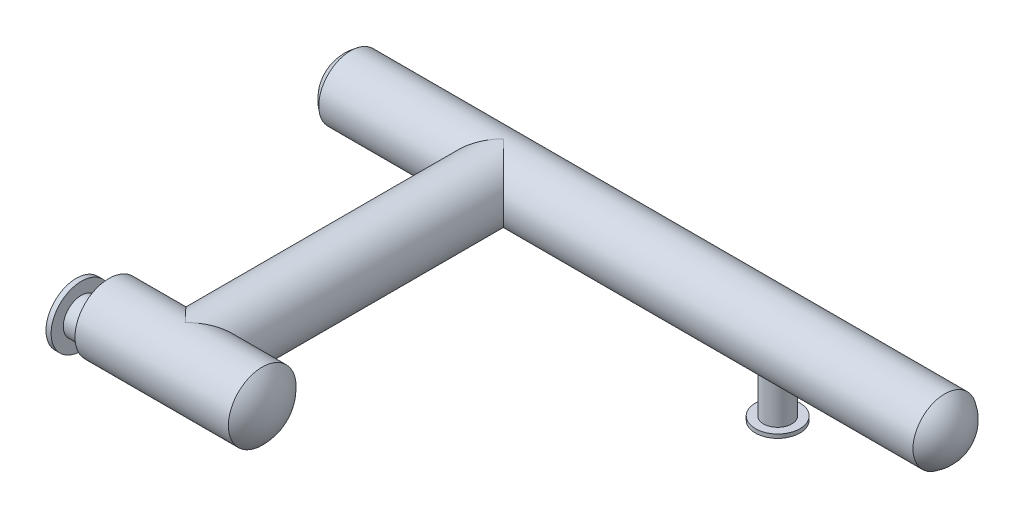
SolidWorks part; units mm, degrees
material "普通碳钢"
ref_plane "Front Plane" through (0, 0, 0) normal (0, 0, 1) x (1, 0, 0)
ref_plane "Top Plane" through (0, 0, 0) normal (0, 1, 0) x (1, 0, 0)
ref_plane "Right Plane" through (0, 0, 0) normal (1, 0, 0) x (0, 0, -1)
sketch "Sketch1" plane through (0, 0, 0) normal (0, 0, 1) x (1, 0, 0)
  line L5 (159.8445, 150) -> (2962.0029, 150)
  line L16 (0, 0) -> (89.3432, 0) construction
  line L17 (79.3432, 0) -> (89.3432, 0)
  line L18 (3047.486, 0) -> (3037.486, 0)
  line L19 (3047.486, 0) -> (2990.0914, 0) construction
  line L20 (162.9067, 140) -> (2959.2196, 140)
  line L21 (96.2314, 0) -> (389.3753, 0) construction
  line L22 (3037.1815, 10) -> (2990.0914, 10) construction
  line L23 (89.6376, 10) -> (96.2314, 10) construction
  line L24 (79.3432, 0) -> (96.2314, 0) construction
  arc A0 (159.8445, 150) -> (79.3432, 0) centre (259.3432, 0) ccw
  arc A1 (2962.0029, 150) -> (3047.486, 0) centre (2873.1395, 0) cw
  arc A2 (2959.2196, 140) -> (3037.486, 0) centre (2873.1395, 0) cw
  arc A3 (162.9067, 140) -> (89.3432, 0) centre (259.3432, 0) ccw
  arc A4 (2959.2196, 140) -> (3037.1815, 10) centre (2873.1395, 0) cw construction
  arc A5 (162.9067, 140) -> (89.6376, 10) centre (259.3432, 0) ccw construction
  dimension "D2" = 180
  dimension "D1" = 10
  dimension "D3" = 150
revolve "Revolve1" add sketch "Sketch1" angle 360 about L16
sketch "Sketch2" plane through (0, 0, 0) normal (0, 0, 1) x (1, 0, 0)
  circle A0 centre (880, 0) radius 150
  circle A1 centre (880, 0) radius 140
  dimension "D1" = 300
  dimension "D2" = 10
extrude "Boss-Extrude1" add sketch "Sketch2" along normal blind 1500
ref_plane "Plane1" through (0, 0, 1500) normal (0, 0, 1) x (1, 0, 0)
sketch "Sketch4" plane through (0, 0, 1500) normal (0, 0, 1) x (1, 0, 0)
  line L1 (1243.1971, 150) -> (519.9222, 150)
  line L2 (2962.0029, 150) -> (880, 150) construction
  line L3 (880, 150) -> (159.8445, 150) construction
  line L4 (496.4048, -9.7617) -> (506.4058, -9.7617)
  line L8 (1239.1001, 140) -> (527.5168, 140)
  line L10 (506.6346, 0.2383) -> (1299.0754, 0.2383) construction
  line L11 (1299.1071, -9.7617) -> (1309.1092, -9.7617)
  line L12 (496.4048, -9.7617) -> (1309.1092, -9.7617) construction
  arc A1 (1309.1092, -9.7617) -> (1243.1971, 150) centre (1093.0729, -5.4133) ccw
  arc A2 (496.4048, -9.7617) -> (519.9222, 150) centre (1110.7572, -18.5847) cw
  arc A3 (506.4058, -9.7617) -> (527.5168, 140) centre (1110.7572, -18.5847) cw
  arc A4 (1299.1071, -9.7617) -> (1239.1001, 140) centre (1093.0729, -5.4133) ccw
  arc A5 (506.6346, 0.2383) -> (527.5168, 140) centre (1110.7572, -18.5847) cw construction
  arc A6 (1299.0754, 0.2383) -> (1239.1001, 140) centre (1093.0729, -5.4133) ccw construction
  dimension "D2" = 10
revolve "Revolve2" add sketch "Sketch4" angle 360 about L4
ref_plane "Plane2" through (550, 0, 0) normal (1, 0, 0) x (0, 0, -1)
sketch "Sketch5" plane through (550, 0, 0) normal (1, 0, 0) x (0, 0, -1)
  circle A0 centre (-1559.9921, -8.7899) radius 85
  circle A1 centre (-1559.9921, -8.7899) radius 79
  circle A2 centre (-1500, -9.7617) radius 159.7617 construction
  dimension "D1" = 170
  dimension "D2" = 6
  dimension "D3" = 60
extrude "Boss-Extrude2" add sketch "Sketch5" against normal blind 100 separate body
sketch "Sketch6" plane through (450, 0, 0) normal (-1, 0, 0) x (0, 0, 1)
  circle A0 centre (1559.9921, -8.7899) radius 60.5
  circle A1 centre (1559.9921, -8.7899) radius 142.5
  dimension "D1" = 285
extrude "Boss-Extrude3" add sketch "Sketch6" along normal blind 24
sketch "Sketch9" plane through (0, 0, 0) normal (0, 1, 0) x (1, 0, 0)
  line L0 (2962.0029, -150) -> (2962.0029, 150) construction
  circle A0 centre (2174.0029, 0) radius 66.5
  circle A1 centre (2174.0029, 0) radius 60.5
  dimension "D1" = 133
  dimension "D2" = 6
  dimension "D3" = 788
extrude "Boss-Extrude4" add sketch "Sketch9" against normal blind 334
sketch "Sketch10" plane through (0, -334, 0) normal (0, -1, 0) x (-1, 0, 0)
  circle A0 centre (-2174.0029, 0) radius 105
  circle A1 centre (-2174.0029, 0) radius 60.5
  dimension "D1" = 210
extrude "Boss-Extrude5" add sketch "Sketch10" along normal blind 18
